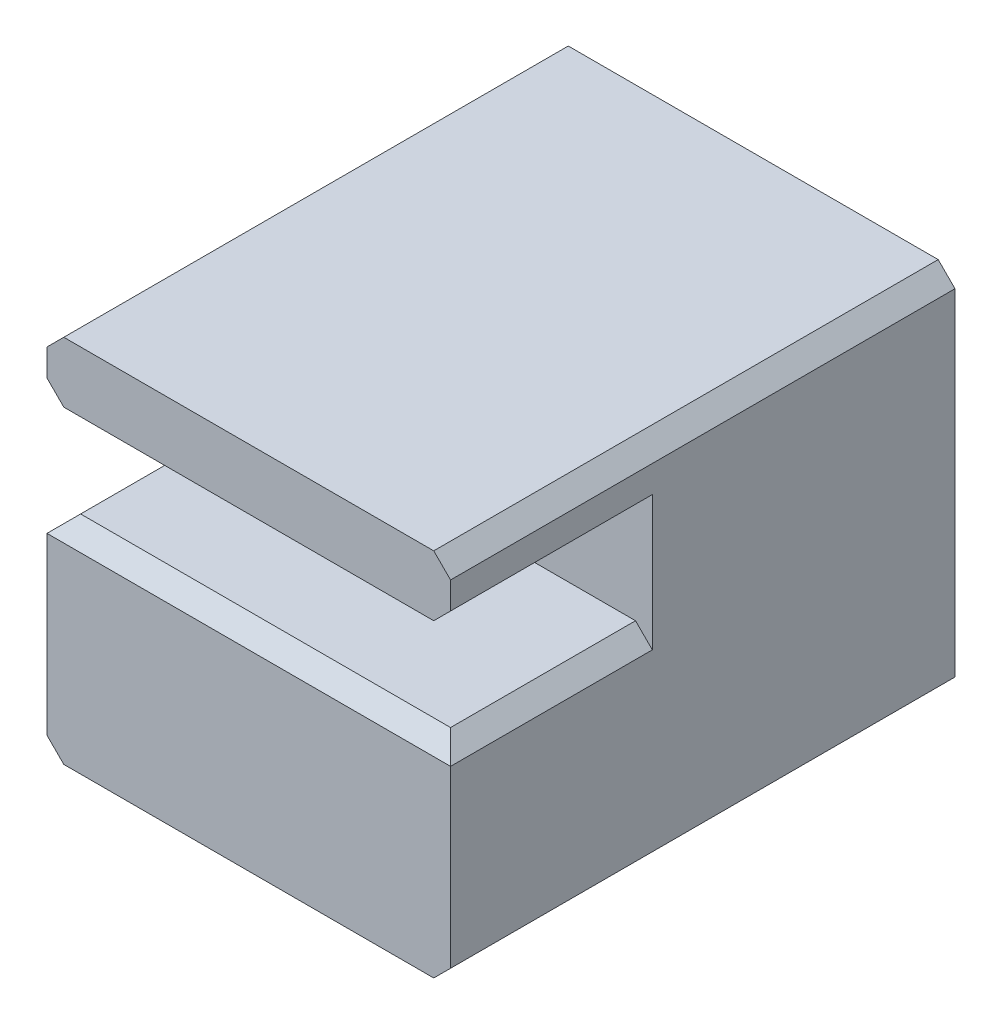
SolidWorks part; units mm, degrees
material "AL6061"
ref_plane "主视基准图" through (0, 0, 0) normal (0, 0, 1) x (1, 0, 0)
ref_plane "上视基准图" through (0, 0, 0) normal (0, 1, 0) x (1, 0, 0)
ref_plane "右视基准图" through (0, 0, 0) normal (1, 0, 0) x (0, 0, -1)
sketch "草图1" plane through (0, 0, 0) normal (0, 0, 1) x (1, 0, 0)
  circle A0 centre (0, 0) radius 8
  dimension "D1" = 16
extrude "凸台-拉伸1" add sketch "草图1" along normal mid plane 15
sketch "草图3" plane through (0, 0, -7.5) normal (0, 0, -1) x (-1, 0, 0)
  circle A0 centre (0, 0) radius 2.5
  dimension "D1" = 5
extrude "切除-拉伸2" cut sketch "草图3" against normal blind 12.5
sketch "草图4" plane through (0, 0, 7.5) normal (0, 0, 1) x (1, 0, 0)
  line L1 (-6, -10.0461) -> (6, -10.0461)
  line L2 (-6, -10.0461) -> (-6, 10.0461)
  line L3 (-6, 10.0461) -> (6, 10.0461)
  line L4 (6, -10.0461) -> (6, 10.0461)
  line L5 (-6, -10.0461) -> (6, 10.0461) construction
  line L6 (-6, 10.0461) -> (6, -10.0461) construction
  point P0 (0, 0)
  dimension "D1" = 12
extrude "切除-拉伸3" cut sketch "草图4" against normal through all flip side to cut
sketch "草图5" plane through (0, 0, 7.5) normal (0, 0, 1) x (1, 0, 0)
  line L1 (-7.8533, -9.3257) -> (8.3323, -9.3257)
  line L2 (-7.8533, -9.3257) -> (-7.8533, -3)
  line L3 (-7.8533, -3) -> (8.3323, -3)
  line L4 (8.3323, -9.3257) -> (8.3323, -3)
  dimension "D1" = 3
extrude "切除-拉伸4" cut sketch "草图5" against normal through all
sketch "草图8" plane through (0, 0, -7.5) normal (0, 0, -1) x (-1, 0, 0)
  line L2 (6, 5.2915) -> (6, -3) construction
  line L3 (-6, 5.2915) -> (6, 5.2915)
  line L4 (-6, 5.2915) -> (-6, 8)
  line L5 (-6, 8) -> (6, 8)
  line L6 (6, 5.2915) -> (6, 8)
  arc A0 (6, 5.2915) -> (-6, 5.2915) centre (0, 0) ccw construction
extrude "凸台-拉伸2" add sketch "草图8" against normal up to surface (15 mm away) up to face at (0, 1.8229, 7.5)
sketch "草图2" plane through (0, 0, 7.5) normal (0, 0, 1) x (1, 0, 0)
  line L7 (-8.2938, 6.2) -> (8.7062, 6.2)
  line L8 (-8.2938, 6.2) -> (-8.2938, 3.2)
  line L9 (-8.2938, 3.2) -> (8.7062, 3.2)
  line L10 (8.7062, 6.2) -> (8.7062, 3.2)
  point P0 (0, 7)
  dimension "D1" = 3.2
  dimension "D2" = 17
  dimension "D3" = 3
chamfer "倒角1" distance 0.5 angle 45 4 edges at (6, -3, 0) (-6, -3, 0) (-6, 8, 0) (6, 8, 0)
extrude "切除-拉伸5" cut sketch "草图2" against normal blind 6
chamfer "倒角2" distance 0.5 angle 45 5 edges at (6, 6.2, 4.5) (-6, 6.2, 4.5) (6, 3.2, 4.5) (0, 3.2, 7.5) (-6, 3.2, 4.5)
